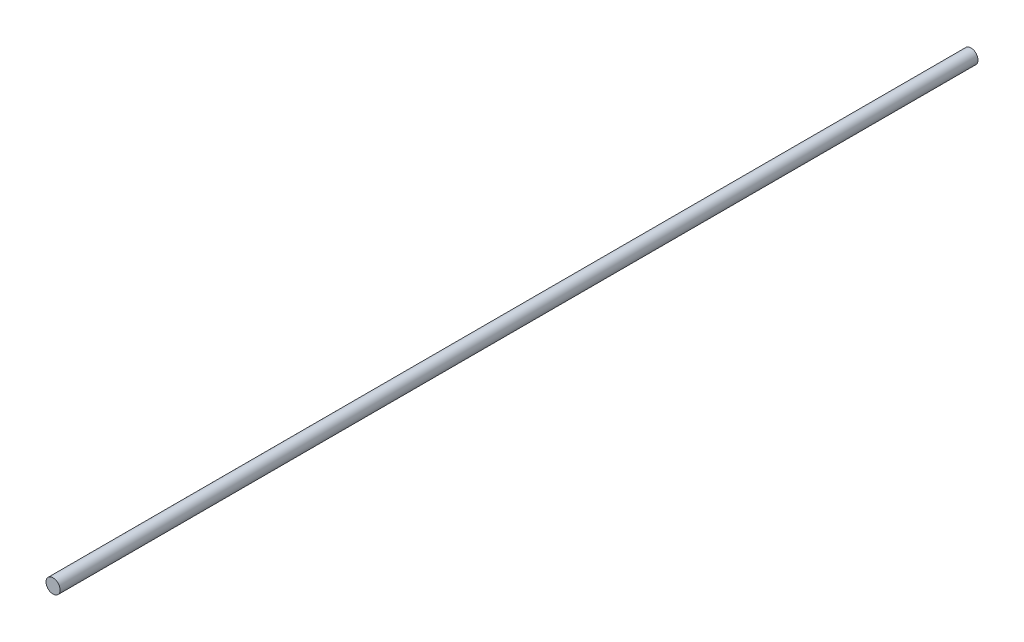
SolidWorks part; units mm, degrees
ref_plane "前视基准面" through (0, 0, 0) normal (0, 0, 1) x (1, 0, 0)
ref_plane "上视基准面" through (0, 0, 0) normal (0, 1, 0) x (1, 0, 0)
ref_plane "右视基准面" through (0, 0, 0) normal (1, 0, 0) x (0, 0, -1)
sketch "草图1" plane through (0, 0, 0) normal (0, 0, 1) x (1, 0, 0)
  circle A0 centre (0, 0) radius 10
  dimension "D1" = 20
extrude "凸台-拉伸1" add sketch "草图1" along normal mid plane 1300
